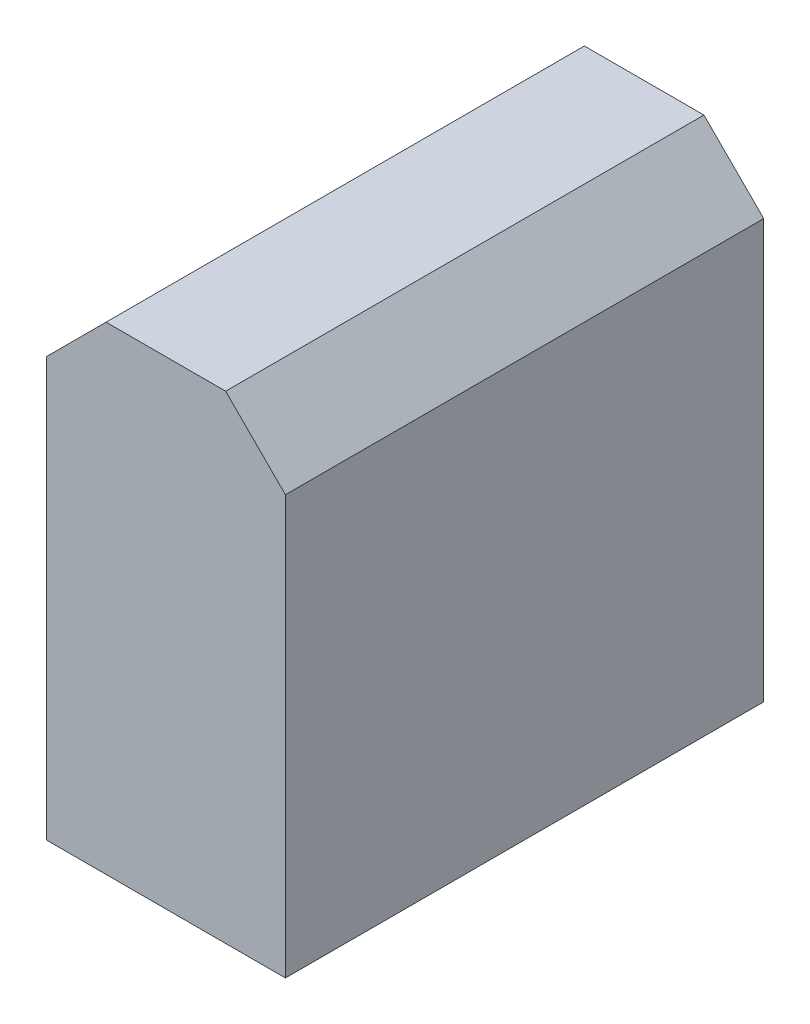
SolidWorks part; units mm, degrees
material "1023 carbon steel plate (SS)"
ref_plane "Front Plane" through (0, 0, 0) normal (0, 0, 1) x (1, 0, 0)
ref_plane "Top Plane" through (0, 0, 0) normal (0, 1, 0) x (1, 0, 0)
ref_plane "Right Plane" through (0, 0, 0) normal (1, 0, 0) x (0, 0, -1)
sketch "Sketch1" plane through (0, 0, 0) normal (0, 0, 1) x (1, 0, 0)
  line L1 (10, 20) -> (-10, 20)
  line L2 (10, 20) -> (10, -20)
  line L3 (10, -20) -> (-10, -20)
  line L4 (-10, 20) -> (-10, -20)
  line L5 (10, 20) -> (-10, -20) construction
  line L6 (10, -20) -> (-10, 20) construction
  point P0 (0, 0)
  dimension "D1" = 20
  dimension "D2" = 40
extrude "Boss-Extrude1" add sketch "Sketch1" along normal blind 40
chamfer "Chamfer1" distance 5 angle 45 2 edges at (-10, 20, 20) (10, 20, 20)
